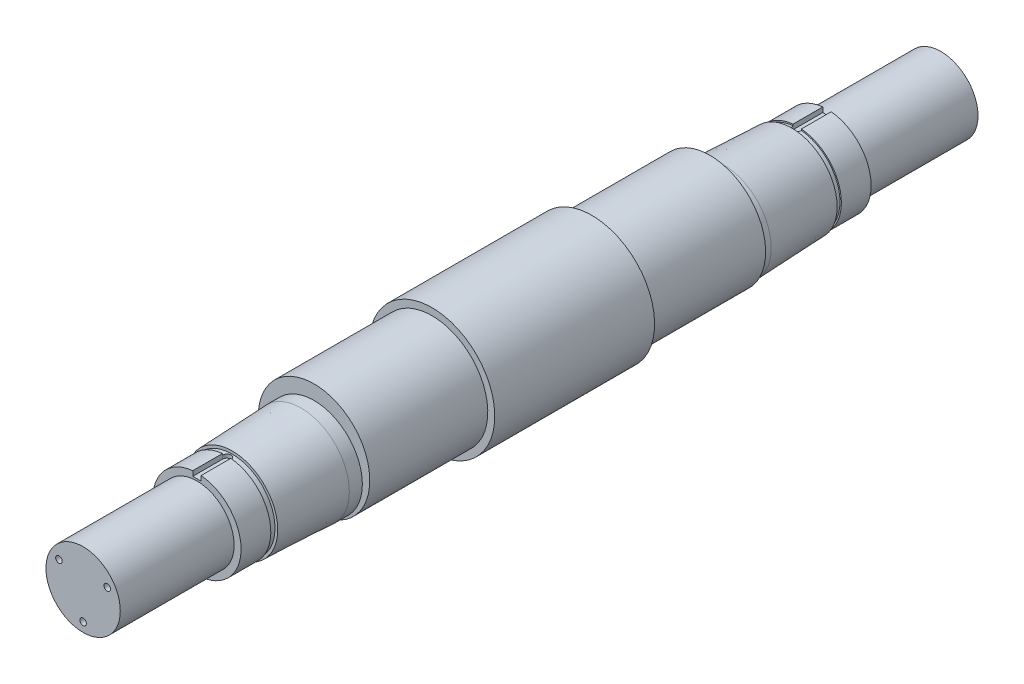
SolidWorks part; units mm, degrees
material "45"
ref_plane "Front Plane" through (0, 0, 0) normal (0, 0, 1) x (1, 0, 0)
ref_plane "Top Plane" through (0, 0, 0) normal (0, 1, 0) x (1, 0, 0)
ref_plane "Right Plane" through (0, 0, 0) normal (1, 0, 0) x (0, 0, -1)
sketch "Sketch2" plane through (0, 0, 0) normal (1, 0, 0) x (0, 0, -1)
  line L0 (-564.378, 0) -> (564.378, 0) construction
  line L1 (0, 0) -> (0, 237.5004) construction
  line L2 (-172, 135) -> (172, 135)
  line L3 (172, 135) -> (172, 120)
  line L4 (172, 120) -> (426, 120)
  line L5 (426, 120) -> (426, 0)
  line L6 (426, 0) -> (0, 0)
  line L7 (0, 0) -> (-426, 0)
  line L8 (-426, 120) -> (-426, 0)
  line L9 (-172, 120) -> (-426, 120)
  line L10 (-172, 135) -> (-172, 120)
  point P4 (0, 0)
  point P10 (0, 10)
  dimension "D1" = 135
  dimension "D2" = 120
  dimension "D3" = 172
  dimension "D4" = 426
revolve "Revolve1" add sketch "Sketch2" angle 360 about L0
sketch "Sketch3" plane through (0, 0, 0) normal (1, 0, 0) x (0, 0, -1)
  line L0 (0, 0) -> (79.8022, 0) construction
  line L1 (0, 0) -> (0, -68.3345) construction
  line L2 (0, -15) -> (690.368, -15) construction
  line L3 (426, -119) -> (426, -15)
  line L5 (426, -120) -> (426, 120) construction
  line L6 (426, -119) -> (454, -119)
  line L7 (454, -119) -> (602, -112.85)
  line L8 (602, -112.85) -> (602, -107)
  line L9 (602, -107) -> (614, -107)
  line L10 (614, -107) -> (614, -110)
  line L11 (614, -110) -> (678, -110)
  line L12 (678, -110) -> (678, -95)
  line L13 (923, -15) -> (426, -15)
  line L14 (678, -95) -> (923, -95)
  line L15 (923, -95) -> (923, -15)
  dimension "D1" = 15
  dimension "D2" = 28
  dimension "D3" = 148
  dimension "D4" = 12
  dimension "D5" = 76
  dimension "D6" = 104
  dimension "D7" = 97.85
  dimension "D8" = 95
  dimension "D9" = 92
  dimension "D10" = 80
  dimension "D11" = 923
revolve "Revolve2" add sketch "Sketch3" angle 360 about L2
mirror "Mirror1" about plane through (0, 0, 0) normal (0, 0, 1) of "Revolve2"
sketch "Sketch5" plane through (0, 0, 0) normal (0, 1, 0) x (1, 0, 0)
  line L0 (0, 0) -> (0, 862.4678) construction
  line L1 (0, 742) -> (0, 614) construction
  line L2 (95, 678) -> (-95, 678) construction
  line L3 (9, 742) -> (9, 614)
  line L4 (-9, 742) -> (-9, 614)
  line L6 (-92, 614) -> (92, 614) construction
  arc A0 (9, 742) -> (-9, 742) centre (0, 742) ccw
  arc A1 (-9, 614) -> (9, 614) centre (0, 614) ccw
  point P7 (0, 678)
  dimension "D1" = 9
extrude "Cut-Extrude3" cut sketch "Sketch5" against normal blind 26.1 from offset 95.1
mirror "Mirror2" about plane through (0, 0, 0) normal (0, 0, 1) of "Cut-Extrude3"
sketch "Sketch6" plane through (0, 0, -923) normal (0, 0, -1) x (-1, 0, 0)
  line L0 (0, -15) -> (51.9615, 15) construction
  line L1 (0, -15) -> (17.6494, -15) construction
  dimension "D1" = 30
  dimension "D2" = 60
hole_wizard "M16 Tapped Hole1" positions "3DSketch1" profile "Sketch7" tap size "M16" standard "GB"
sketch3d "3DSketch1"
  point P0 (-51.9615, 15, -923)
sketch "Sketch7" plane through (-51.9615, 15, -923) normal (1, 0, 0) x (0, 1, 0)
  line L0 (0, 0) -> (0, 42.206)
  line L1 (0, 42.206) -> (7, 38)
  line L2 (7, 38) -> (7, 0)
  line L5 (7, 0) -> (0, 0)
  line L10 (0, 42.206) -> (-7, 38) construction
  line L11 (0, -6.35) -> (0, 107.95) construction
  dimension "螺纹孔钻头直径" = 14
  dimension "螺纹孔钻头深度" = 38
  dimension "导头角度" = 118
cosmetic thread "hole cosmetic thread 1" parameters "D1"=32, "D2"=16
pattern_circular "CirPattern1" count 3 over 360 about axis through (0, -15, 0) along (0, 0, 1) of "M16 Tapped Hole1"
mirror "Mirror3" about plane through (0, 0, 0) normal (0, 0, 1) of "CirPattern1", "M16 Tapped Hole1"
